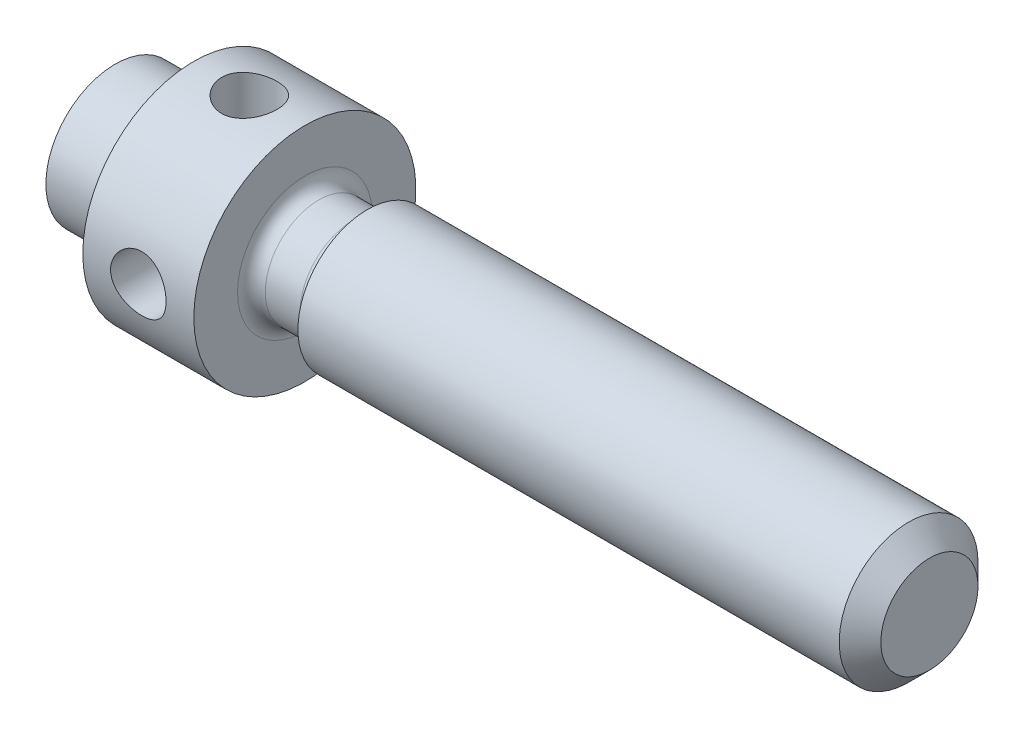
SolidWorks part; units mm, degrees
material "Nickel"
ref_plane "Front" through (0, 0, 0) normal (0, 0, 1) x (1, 0, 0)
ref_plane "Top" through (0, 0, 0) normal (0, 1, 0) x (1, 0, 0)
ref_plane "Right" through (0, 0, 0) normal (1, 0, 0) x (0, 0, -1)
sketch "Sketch1" plane through (0, 0, 0) normal (1, 0, 0) x (0, 0, -1)
  line L0 (-44.7783, 0) -> (45.191, 0) construction
  line L1 (0, 40.8576) -> (0, -40.0322) construction
  circle A0 centre (0, 0) radius 5
  point P7 (9.9873, 7.697)
  point P8 (6.1225, 10.002)
  point P9 (28.4898, 49.0495)
extrude "Boss-Extrude" add sketch "Sketch1" against normal blind 40.5
chamfer "Chamfer2" distance 1.5 1 edges at (0, 0, -5)
sketch "Sketch2" plane through (-40.5, 0, 0) normal (-1, 0, 0) x (0, 0, 1)
  circle A0 centre (0, 0) radius 3.85
  dimension "d3" = 7.7
extrude "Boss-Extrude1" add sketch "Sketch2" along normal blind 4.5
sketch "Sketch4" plane through (-45, 0, 0) normal (-1, 0, 0) x (0, 0, 1)
  circle A0 centre (0, 0) radius 8
  dimension "D" = 16
extrude "Boss-Extrude2" add sketch "Sketch4" along normal blind 8
ref_plane "Plane1" through (-49, 0, 0) normal (1, 0, 0) x (0, 0, -1)
sketch "Sketch5" plane through (-49, 0, 0) normal (1, 0, 0) x (0, 0, -1)
  line L0 (-6.2555, 0) -> (5.9656, 0) construction
  line L1 (0, 6.0883) -> (0, -6.4674) construction
sketch "Sketch6" plane through (0, 0, 0) normal (0, 0, 1) x (1, 0, 0)
  circle A0 centre (-49, 0) radius 2
  dimension "d2" = 4
extrude "Cut-Extrude1" cut sketch "Sketch6" against normal through all and the other way through all
sketch "Sketch7" plane through (0, 0, 0) normal (0, 1, 0) x (1, 0, 0)
  circle A0 centre (-49, 0) radius 2
  dimension "d2" = 4
extrude "Cut-Extrude2" cut sketch "Sketch7" against normal through all and the other way through all
sketch "Sketch12" plane through (-53, 0, 0) normal (-1, 0, 0) x (0, 0, 1)
  line L0 (-6.6686, 0) -> (6.7985, 0) construction
  line L1 (0, 0) -> (8, 0) construction
  line L2 (0, 6.744) -> (0, -6.1631) construction
  line L3 (0, 0) -> (0, 7.746) construction
  line L4 (0, 6.0883) -> (0, -6.4674) construction
sketch "Sketch14" plane through (0, 0, 0) normal (0, 0, 1) x (1, 0, 0)
  line L0 (-53, 0) -> (-53, 5)
  line L1 (-53, 6.744) -> (-53, -6.1631) construction
  line L2 (-53, 5) -> (-58.6603, 5)
  line L3 (-53, 0) -> (-60, 0) construction
  line L4 (-53, 0) -> (-60, 0)
  line L5 (-53, 8) -> (-53, -8) construction
  line L6 (-25.6268, 0) -> (0.8875, 0) construction
  line L7 (-40.5, 0) -> (-1.5, 0) construction
  arc A0 (-58.6603, 5) -> (-60, 0) centre (-50, 0) ccw
  dimension "d1" = 10
  dimension "d1/2" = 5
  dimension "L-lx-H" = 7
revolve "Boss-Revolve1" add sketch "Sketch14" angle 360 about L3
fillet "Fillet1" radius 1 2 edges at (-40.5, 0, -3.85) (-45, 0, 3.85)
sketch "Sketch15" plane through (0, 0, 0) normal (0, 1, 0) x (1, 0, 0)
  line L1 (-58.6603, 5) -> (-68.9851, 5)
  line L2 (-58.6603, 5) -> (-58.6603, -9.8344)
  line L3 (-58.6603, -9.8344) -> (-68.9851, -9.8344)
  line L4 (-68.9851, 5) -> (-68.9851, -9.8344)
extrude "Cut-Extrude3" cut sketch "Sketch15" against normal mid plane 43
equation "\"b@Boss-Extrude1\" = \"b@Sketch1\""
equation "\"lx-b@Boss-Extrude\" = \"length@Sketch1\" - \"b@Sketch1\""
